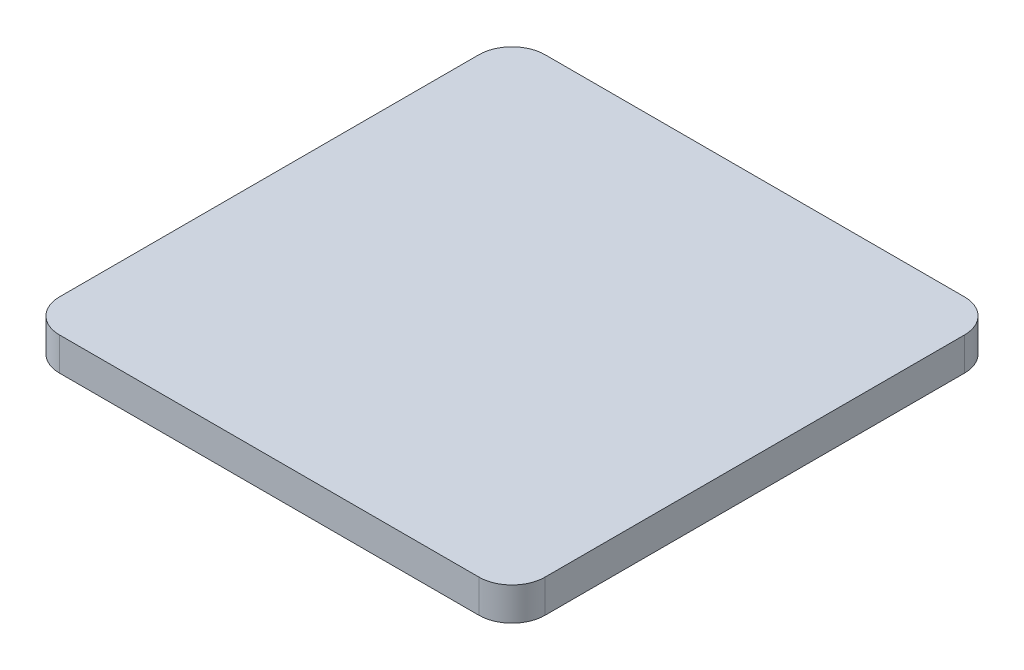
from build123d import *

# Parameters (mm, degrees)
SKETCH_1_W      = 44
SKETCH_1_H      = 44
EXTRUDE_1_DEPTH = 3
FILLET_1_R      = 3


with BuildPart() as part:
    # 草图1 → 凸台-拉伸1 (new body)
    with BuildSketch(Plane(origin=(0, 0, 0), x_dir=(1, 0, 0), z_dir=(0, 1, 0))):
        Rectangle(SKETCH_1_W, SKETCH_1_H)
    extrude(amount=EXTRUDE_1_DEPTH)

    # 圆角1
    fillet_1_edges = [part.edges().sort_by_distance(p)[0] for p in [
        (22, 1.5, 22),
        (-22, 1.5, 22),
        (-22, 1.5, -22),
        (22, 1.5, -22),
    ]]
    fillet(fillet_1_edges, radius=FILLET_1_R)


solid = part.part
